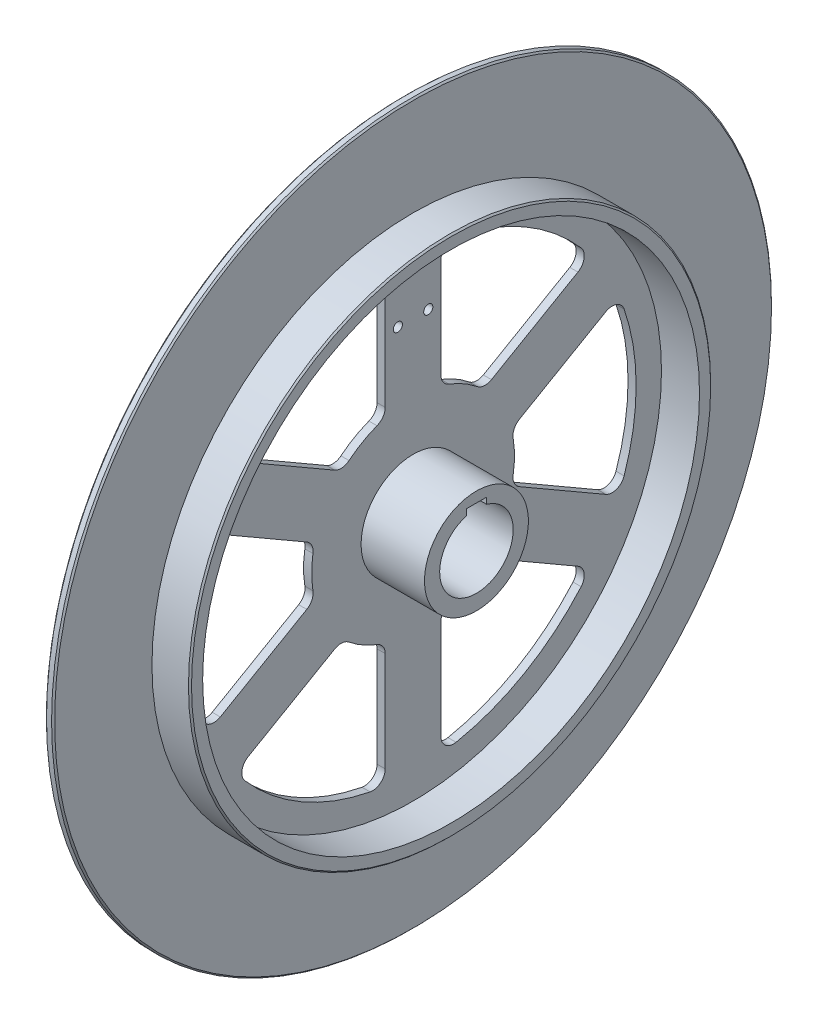
from build123d import *

# Parameters (mm, degrees)
CUT_EXTRUDE1_DEPTH       = 1014.9432923
CIRPATTERN1_COUNT        = 6
BOSS_EXTRUDE1_REACH      = 1015.943
FILLET2_R                = 10
CIRPATTERN2_COUNT        = 6
FILLET2_OF_CIRPATTERN2_R = 10
SKETCH5_R                = 9
CUT_EXTRUDE2_DEPTH       = 1014.9432923
CUT_EXTRUDE3_DEPTH       = 20
CUT_EXTRUDE3_DEPTH_BACK  = 1041.251892572
CHAMFER1_SIZE            = 3
SKETCH7_W                = 40
SKETCH7_H                = 18.8
CUT_EXTRUDE4_DEPTH       = 1035.746345729


with BuildPart() as part:
    # Sketch1 → Revolve1 (revolve)
    with BuildSketch(Plane.XY, mode=Mode.PRIVATE) as revolve1_sk:
        Polygon((0, 102.5), (79, 102.5), (79, 137.5), (109, 137.5), (109, 534), (-31, 534), (-31, 550), (109, 550), (109, 710), (125, 710), (125, 515), (200, 515), (200, 490), (125, 490), (125, 102.5), (250, 102.5), (250, 72.5), (0, 72.5), align=None)
    revolve(revolve1_sk.sketch.rotate(Axis((-373.351674541, 0, 0), (1, 0, 0)), 90), axis=Axis((-373.351674541, 0, 0), (1, 0, 0)))

    # Sketch3 → Cut-Extrude1 (cut, through all)
    with BuildSketch(Plane.ZY.offset(-109)):
        with BuildLine():
            Line((-55, 407.216158815), (-55, 210.297408448))
            ThreePointArc((-55, 210.297408448), (-59.418184941, 196.106253143), (-71.111111111, 186.931029732))
            ThreePointArc((-71.111111111, 186.931029732), (-100, 173.205080757), (-126.331464948, 155.049543579))
            ThreePointArc((-126.331464948, 155.049543579), (-140.123904592, 149.510784178), (-154.622898066, 152.780101432))
            Line((-154.622898066, 152.780101432), (-325.159538365, 251.239476616))
            ThreePointArc((-325.159538365, 251.239476616), (-337.320790629, 268.78857093), (-331.494450315, 289.329275066))
            ThreePointArc((-331.494450315, 289.329275066), (-220, 381.051177665), (-84.819277108, 431.747252719))
            ThreePointArc((-84.819277108, 431.747252719), (-64.117335358, 426.522659374), (-55, 407.216158815))
        make_face()
    cut_extrude1 = extrude(amount=-CUT_EXTRUDE1_DEPTH, mode=Mode.SUBTRACT)

    # CirPattern1: Cut-Extrude1 ×6 about axis
    cirpattern1_axis = Axis((0, 0, 0), (1, 0, 0))
    for i in range(1, CIRPATTERN1_COUNT):
        add(cut_extrude1.rotate(cirpattern1_axis, i * 360 / CIRPATTERN1_COUNT), mode=Mode.SUBTRACT)

    # Boss-Extrude1: up to this face of the body (flat: up to its plane)
    boss_extrude1_end = Plane(part.part.faces().sort_by_distance((0, 0, -75.399137803))[0])
    # Sketch4 → Boss-Extrude1 (add, up to the picked face)
    with BuildSketch(Plane.ZY.offset(-109), mode=Mode.PRIVATE) as boss_extrude1_sk1:
        with BuildLine():
            Line((-8, 533.940071544), (-8, 102.187327982))
            ThreePointArc((-8, 102.187327982), (0, 102.5), (8, 102.187327982))
            Line((8, 102.187327982), (8, 533.940071544))
            ThreePointArc((8, 533.940071544), (0, 534), (-8, 533.940071544))
        make_face()
    boss_extrude1_tool1 = split(extrude(boss_extrude1_sk1.sketch, amount=BOSS_EXTRUDE1_REACH, mode=Mode.PRIVATE), bisect_by=boss_extrude1_end, keep=Keep.BOTH, mode=Mode.PRIVATE)
    boss_extrude1 = boss_extrude1_tool1.solids().sort_by(Axis((109, 318.187922, 0), (-1, 0, 0)))[0]
    add(boss_extrude1)

    # Fillet2
    fillet2_edges = [part.edges().sort_by_distance(p)[0] for p in [
        (94, 137.267075441, 8),
        (39.5, 102.187327982, -8),
        (94, 137.267075441, -8),
        (109, 335.603573492, 8),
        (39.5, 102.187327982, 8),
        (54.5, 533.940071544, -8),
        (109, 335.603573492, -8),
        (54.5, 533.940071544, 8),
    ]]
    fillet(fillet2_edges, radius=FILLET2_R)

    # CirPattern2: Boss-Extrude1 ×6 about axis
    cirpattern2_axis = Axis((0, 0, 0), (1, 0, 0))
    for i in range(1, CIRPATTERN2_COUNT):
        add(boss_extrude1.rotate(cirpattern2_axis, i * 360 / CIRPATTERN2_COUNT))

    # Fillet2 of CirPattern2
    fillet2_of_cirpattern2_edges = [part.edges().sort_by_distance(p)[0] for p in [
        (94, 61.70533449, 122.876774435),
        (39.5, 58.021867221, 84.496821977),
        (94, 75.561740951, 114.876774435),
        (109, 160.873583516, 294.641220245),
        (39.5, 44.16546076, 92.496821977),
        (54.5, 273.898239002, 458.405666055),
        (109, 174.729989976, 286.641220245),
        (54.5, 260.041832542, 466.405666055),
        (94, -75.561740951, 114.876774435),
        (39.5, -44.16546076, 92.496821977),
        (94, -61.70533449, 122.876774435),
        (109, -174.729989976, 286.641220245),
        (39.5, -58.021867221, 84.496821977),
        (54.5, -260.041832542, 466.405666055),
        (109, -160.873583516, 294.641220245),
        (54.5, -273.898239002, 458.405666055),
        (94, -137.267075441, -8),
        (39.5, -102.187327982, 8),
        (94, -137.267075441, 8),
        (109, -335.603573492, -8),
        (39.5, -102.187327982, -8),
        (54.5, -533.940071544, 8),
        (109, -335.603573492, 8),
        (54.5, -533.940071544, -8),
        (94, -61.70533449, -122.876774435),
        (39.5, -58.021867221, -84.496821977),
        (94, -75.561740951, -114.876774435),
        (109, -160.873583516, -294.641220245),
        (39.5, -44.16546076, -92.496821977),
        (54.5, -273.898239002, -458.405666055),
        (109, -174.729989976, -286.641220245),
        (54.5, -260.041832542, -466.405666055),
        (94, 75.561740951, -114.876774435),
        (39.5, 44.16546076, -92.496821977),
        (94, 61.70533449, -122.876774435),
        (109, 174.729989976, -286.641220245),
        (39.5, 58.021867221, -84.496821977),
        (54.5, 260.041832542, -466.405666055),
        (109, 160.873583516, -294.641220245),
        (54.5, 273.898239002, -458.405666055),
    ]]
    fillet(fillet2_of_cirpattern2_edges, radius=FILLET2_OF_CIRPATTERN2_R)

    # Sketch5 → Cut-Extrude2 (cut, through all)
    with BuildSketch(Plane.ZY.offset(-109)):
        with Locations((-30, 425)):
            Circle(SKETCH5_R)
        with Locations((-30, 335)):
            Circle(SKETCH5_R)
        with Locations((30, 335)):
            Circle(SKETCH5_R)
        with Locations((30, 425)):
            Circle(SKETCH5_R)
    extrude(amount=-CUT_EXTRUDE2_DEPTH, mode=Mode.SUBTRACT)

    # Sketch6 → Cut-Extrude3 (cut, two sides: drawn at the far end of the back side and taken through both)
    with BuildSketch(Plane.XY.offset(8).offset(-CUT_EXTRUDE3_DEPTH_BACK)):
        with BuildLine():
            Line((94, 395), (109, 395))
            Line((109, 395), (109, 365))
            Line((109, 365), (94, 365))
            ThreePointArc((94, 365), (79, 380), (94, 395))
        make_face()
    extrude(amount=CUT_EXTRUDE3_DEPTH + CUT_EXTRUDE3_DEPTH_BACK, mode=Mode.SUBTRACT)

    # Chamfer1
    chamfer1_edges = [part.edges().sort_by_distance(p)[0] for p in [
        (-31, 0, -550),
        (109, 0, -710),
        (125, 0, -710),
        (200, 0, -515),
    ]]
    chamfer(chamfer1_edges, length=CHAMFER1_SIZE)

    # Sketch7 → Cut-Extrude4 (cut, through all)
    with BuildSketch(Plane.ZY):
        with Locations((0, 72.5)):
            Rectangle(SKETCH7_W, SKETCH7_H)
    extrude(amount=-CUT_EXTRUDE4_DEPTH, mode=Mode.SUBTRACT)

    # Sketch8 → Cut-Revolve1 (revolve, cut)
    with BuildSketch(Plane.XY, mode=Mode.PRIVATE) as cut_revolve1_sk:
        Polygon((109, 550), (-31, 550), (-31, 146.397575117), (-31, 0), (49, 0), (49, 101.17949397), (79, 101.17949397), (79, 136.472315787), (109, 136.472315787), align=None)
    revolve(cut_revolve1_sk.sketch.rotate(Axis((0, 0, 0), (-1, 0, 0)), 90), axis=Axis((0, 0, 0), (-1, 0, 0)), mode=Mode.SUBTRACT)


solid = part.part
